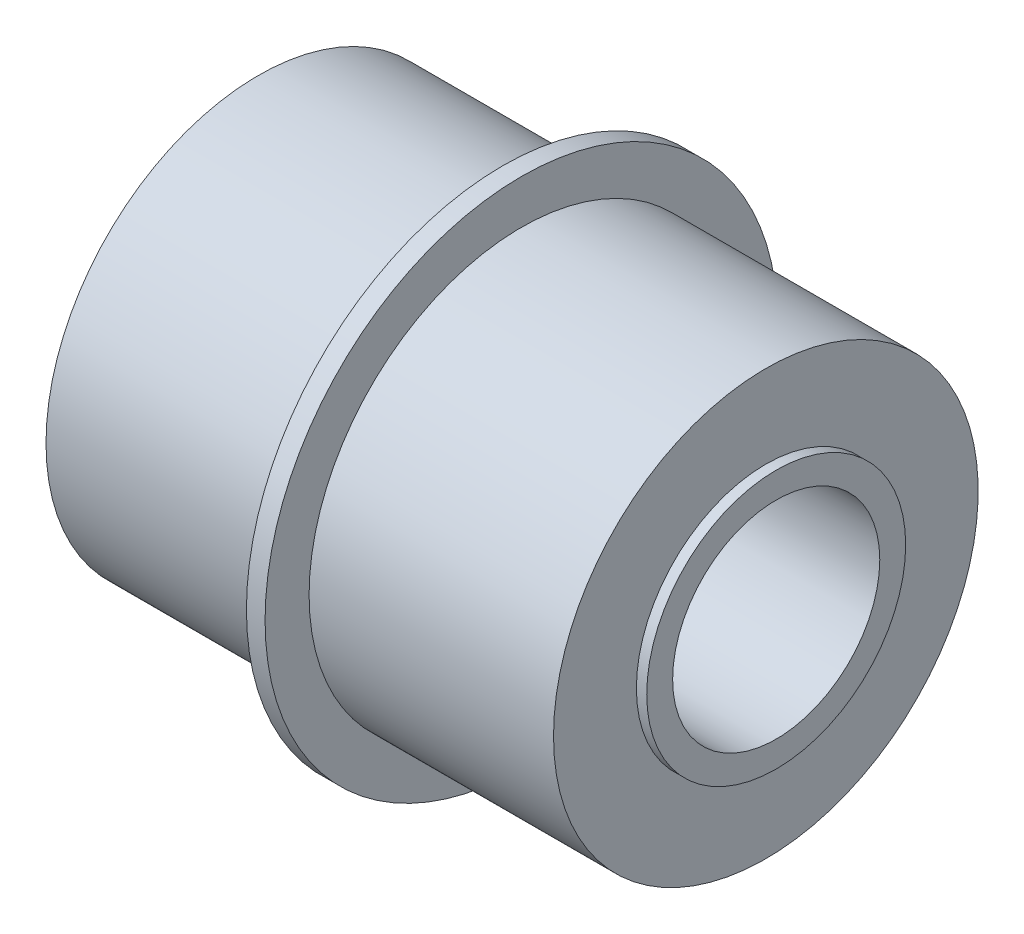
from build123d import *


with BuildPart() as part:
    # 草图1 → 旋转1 (revolve)
    with BuildSketch(Plane.XY, mode=Mode.PRIVATE) as revolve_1_sk:
        Polygon((-0.9, 24.75), (0.9, 24.75), (0.9, 20.5), (24.5, 20.5), (24.5, 12.5), (25.5, 12.5), (25.5, 10), (-25.5, 10), (-25.5, 12.5), (-24.5, 12.5), (-24.5, 20.5), (-0.9, 20.5), align=None)
    revolve(revolve_1_sk.sketch.rotate(Axis((-73.221991318, 0, 0), (1, 0, 0)), 90), axis=Axis((-73.221991318, 0, 0), (1, 0, 0)))


solid = part.part
